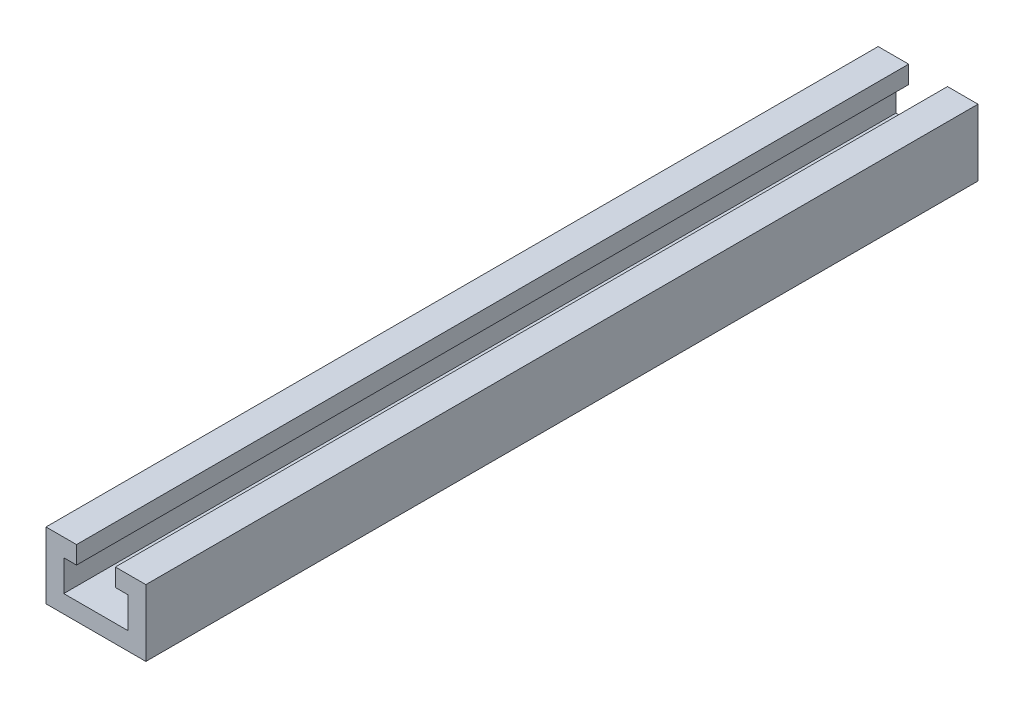
from build123d import *

# Parameters (mm, degrees)
EXTRUDE_1_DEPTH = 37.5


with BuildPart() as part:
    # 草图1 → 凸台-拉伸1 (new, symmetric)
    with BuildSketch(Plane.XY):
        Polygon((0, 0), (-4.5, 0), (-4.5, 6), (-1.75, 6), (-1.75, 4.4), (-2.9, 4.4), (-2.9, 1.6), (2.9, 1.6), (2.9, 4.4), (1.75, 4.4), (1.75, 6), (4.5, 6), (4.5, 0), align=None)
    extrude(amount=EXTRUDE_1_DEPTH, both=True)


solid = part.part
